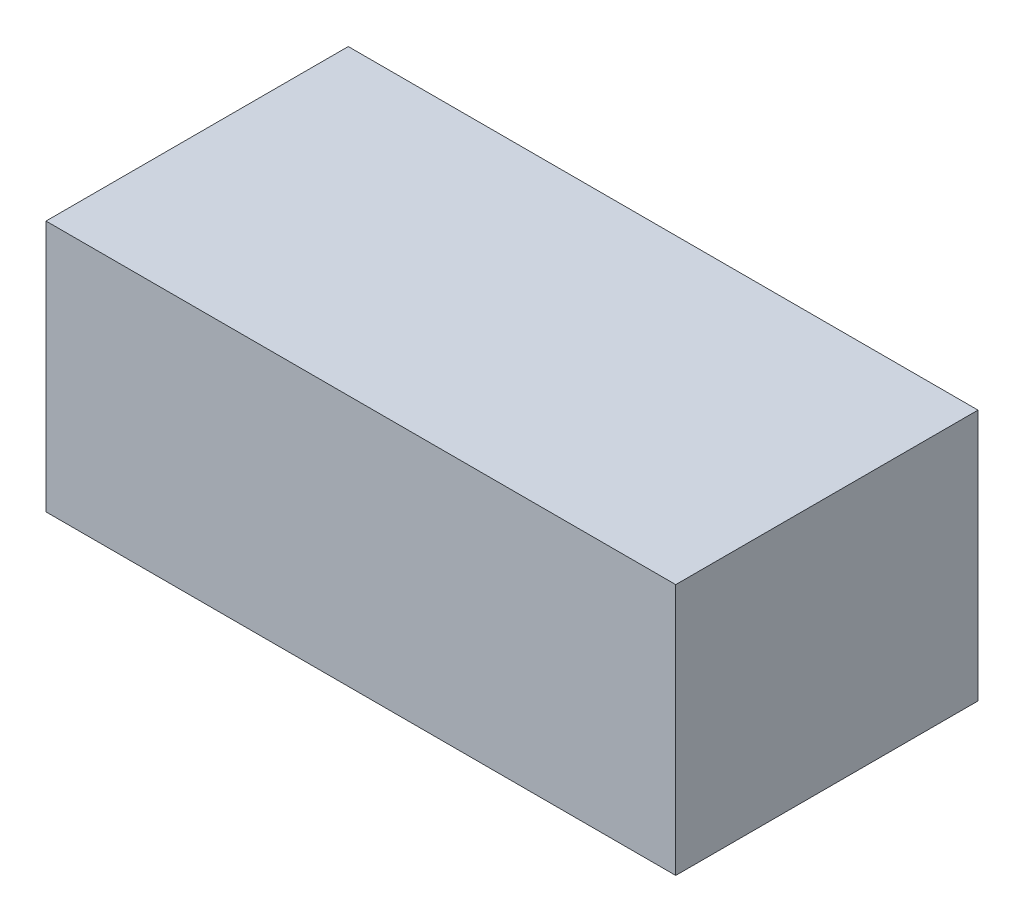
from build123d import *

# Parameters (mm, degrees)
SKETCH_1_W      = 25
SKETCH_1_H      = 10
EXTRUDE_1_DEPTH = 6


with BuildPart() as part:
    # 草图1 → 凸台-拉伸1 (new, symmetric)
    with BuildSketch(Plane.XY):
        Rectangle(SKETCH_1_W, SKETCH_1_H)
    extrude(amount=EXTRUDE_1_DEPTH, both=True)


solid = part.part
